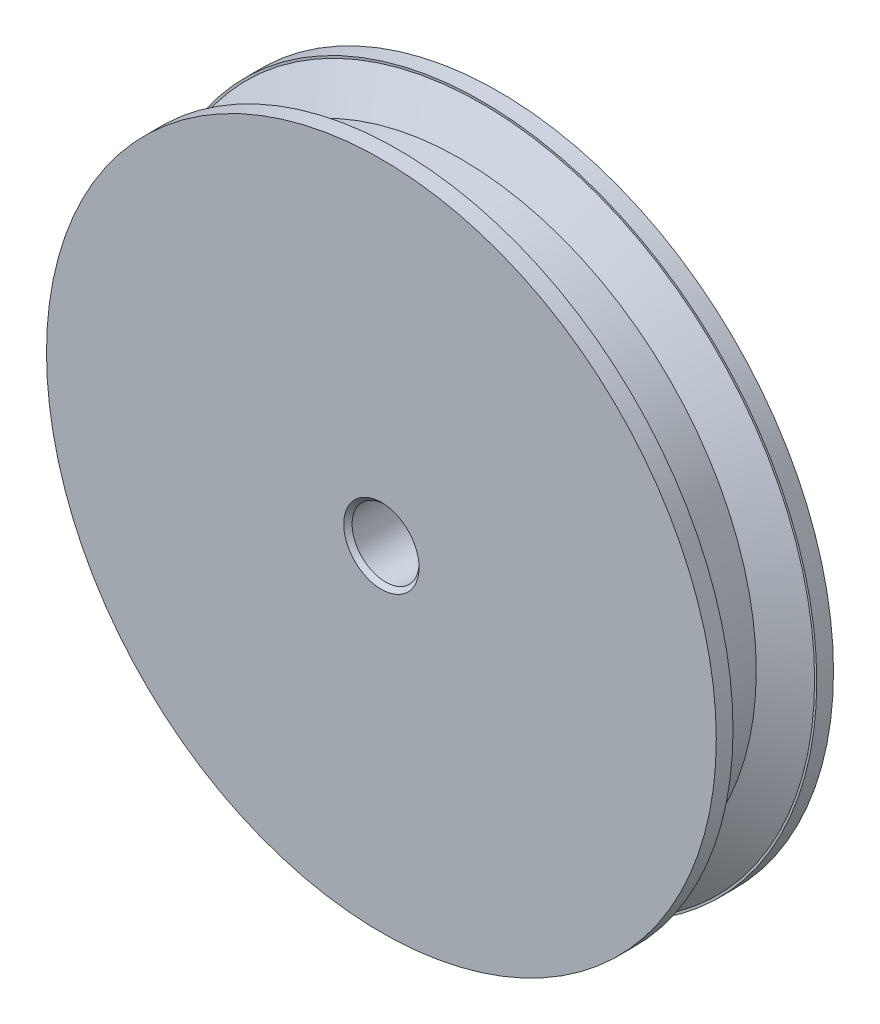
from build123d import *

# Parameters (mm, degrees)
SKETCH1_R           = 40
SKETCH1_R_2         = 4
BOSS_EXTRUDE1_DEPTH = 7
CHAMFER1_SIZE       = 0.5


with BuildPart() as part:
    # Sketch1 → Boss-Extrude1 (new, symmetric)
    with BuildSketch(Plane.XY):
        Circle(SKETCH1_R)
        Circle(SKETCH1_R_2, mode=Mode.SUBTRACT)
    extrude(amount=BOSS_EXTRUDE1_DEPTH, both=True)

    # Sketch2 → Cut-Revolve1 (revolve, cut)
    with BuildSketch(Plane(origin=(0, 0, 0), x_dir=(0, 0, -1), z_dir=(1, 0, 0)), mode=Mode.PRIVATE) as cut_revolve1_sk:
        Polygon((-5, 39.744407704), (-2.448600638, 35.325254378), (2.448600638, 35.325254378), (5, 39.744407704), (5, 40), (-5, 40), align=None)
    revolve(cut_revolve1_sk.sketch.rotate(Axis((0, 0, 7), (0, 0, -1)), 90), axis=Axis((0, 0, 7), (0, 0, -1)), mode=Mode.SUBTRACT)

    # Chamfer1
    chamfer1_edges = [part.edges().sort_by_distance(p)[0] for p in [
        (-4, 0, -7),
        (-4, 0, 7),
    ]]
    chamfer(chamfer1_edges, length=CHAMFER1_SIZE)


solid = part.part
